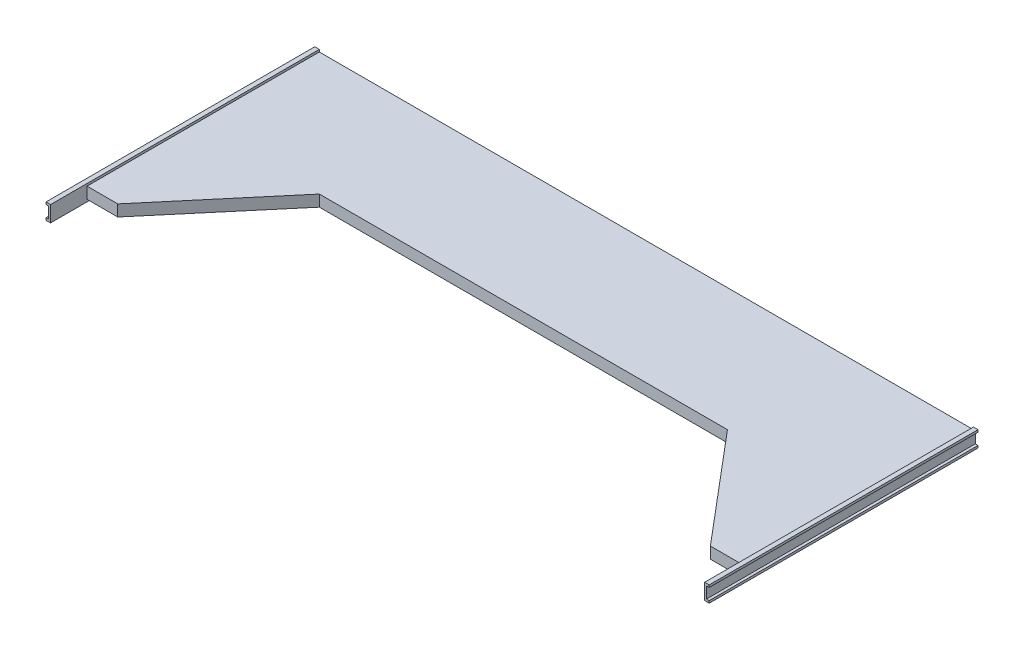
from build123d import *

# Parameters (mm, degrees)
BOSS_EXTRUDE1_DEPTH = 590
CUT_EXTRUDE1_REACH  = 1573.285


with BuildPart() as part:
    # Sketch1 → Boss-Extrude1 (new body)
    with BuildSketch(Plane.XY):
        Polygon((10, 25), (10, 30), (0, 30), (0, 25), (5, 25), (5, 0), (0, 0), (0, -5), (10, -5), (10, 0), (1446, 0), (1446, -5), (1456, -5), (1456, 0), (1450, 0), (1450, 25), (1456, 25), (1456, 30), (1446, 30), (1446, 25), align=None)
    extrude(amount=BOSS_EXTRUDE1_DEPTH)

    # Sketch2 → Cut-Extrude1 (cut, up to next)
    with BuildSketch(Plane(origin=(0, 25, 0), x_dir=(1, 0, 0), z_dir=(0, 1, 0)), mode=Mode.PRIVATE) as cut_extrude1_sk1:
        Polygon((10, -590), (1446, -590), (1446, -510), (1378.5, -510), (1176, -270), (280, -270), (77.5, -510), (10, -510), align=None)
    cut_extrude1_tool1 = extrude(cut_extrude1_sk1.sketch, amount=-CUT_EXTRUDE1_REACH, mode=Mode.PRIVATE) & part.part
    add(cut_extrude1_tool1.solids().sort_by_distance((728, 25, 443.695445))[0], mode=Mode.SUBTRACT)


solid = part.part
